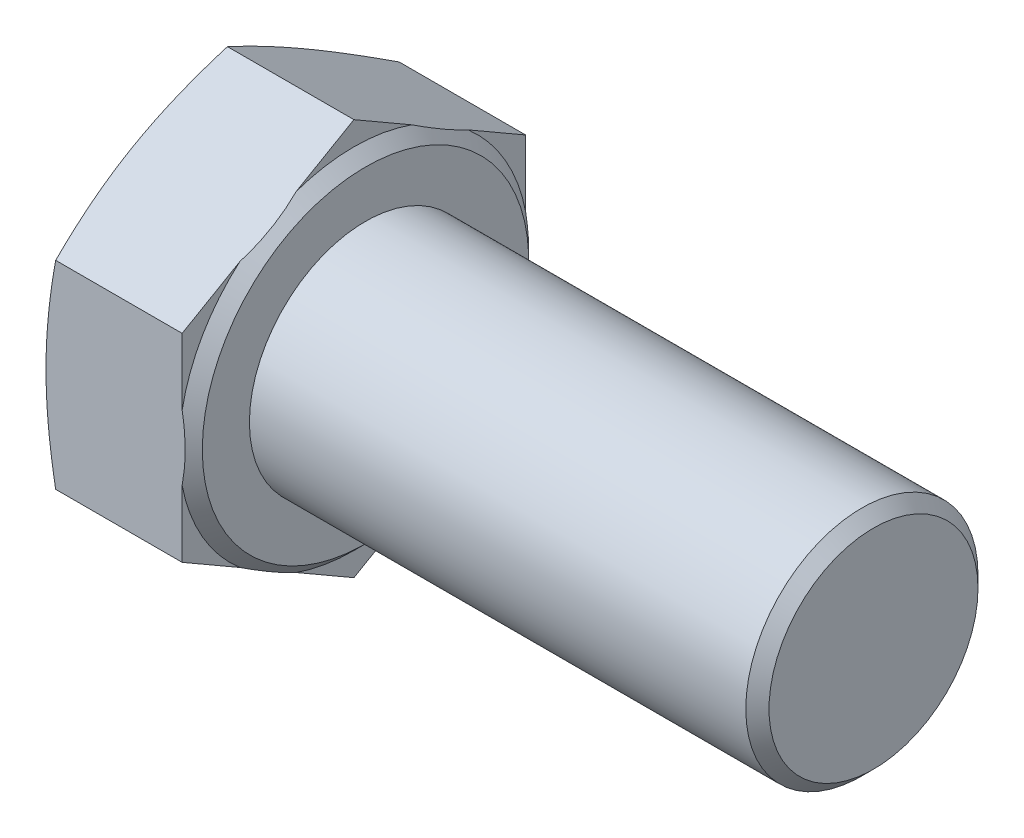
from build123d import *

# Parameters (mm, degrees)
BASEHEAD_DEPTH = 10.18
SKETCH5_R      = 8
BASEBODY_DEPTH = 35
CHAMFER1_SIZE  = 0.8


with BuildPart() as part:
    # Sketch2 → BaseHead (new body)
    with BuildSketch(Plane(origin=(0, 0, 0), x_dir=(0, 0, -1), z_dir=(1, 0, 0))):
        Polygon((11.835, -6.832940436), (11.835, 6.832940436), (0, 13.665880872), (-11.835, 6.832940436), (-11.835, -6.832940436), (0, -13.665880872), align=None)
    extrude(amount=BASEHEAD_DEPTH)

    # Sketch3 → BearingFace (revolve, cut)
    with BuildSketch(Plane.XY, mode=Mode.PRIVATE) as bearingface_sk:
        Polygon((10.18, 13.665880872), (10.18, 11.245), (9.38, 12.045), (9.38, 13.665880872), align=None)
    revolve(bearingface_sk.sketch.rotate(Axis((-0.957090588, 0, 0), (1, 0, 0)), 90), axis=Axis((-0.957090588, 0, 0), (1, 0, 0)), mode=Mode.SUBTRACT)

    # Sketch4 → HeadChamfer (revolve, cut)
    with BuildSketch(Plane.XY):
        Polygon((0, 13.665880872), (0.66638614, 13.665880872), (0, 11.835), align=None)
    revolve(axis=Axis((-0.493528746, 0, 0), (1, 0, 0)), mode=Mode.SUBTRACT)

    # Sketch5 → BaseBody (add)
    with BuildSketch(Plane(origin=(10.18, 0, 0), x_dir=(0, 0, -1), z_dir=(1, 0, 0))):
        with Locations(Location((0, 0, 0), (0, 0, 180))):
            Circle(SKETCH5_R)
    extrude(amount=BASEBODY_DEPTH)

    # Chamfer1
    chamfer1_edges = [part.edges().sort_by_distance(p)[0] for p in [
        (45.18, 0, -8),
    ]]
    chamfer(chamfer1_edges, length=CHAMFER1_SIZE)


solid = part.part
